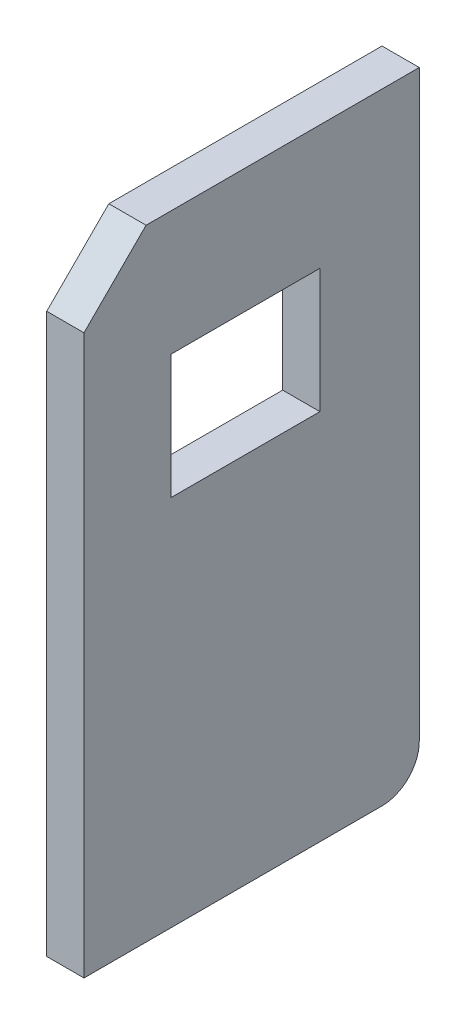
from build123d import *

# Parameters (mm, degrees)
EXTRUDE_1_DEPTH     = 3
FILLET_1_R          = 3
SKETCH_2_W          = 12
SKETCH_2_H          = 10
CUT_EXTRUDE_1_DEPTH = 57.903426962


with BuildPart() as part:
    # 草图1 → 凸台-拉伸1 (new body)
    with BuildSketch(Plane(origin=(0, 0, 0), x_dir=(0, 0, -1), z_dir=(1, 0, 0))):
        Polygon((-22, 50), (-27, 45), (-27, 0), (0, 0), (0, 50), align=None)
    extrude(amount=EXTRUDE_1_DEPTH)

    # 圆角1
    fillet_1_edges = [part.edges().sort_by_distance(p)[0] for p in [
        (1.5, 0, 0),
    ]]
    fillet(fillet_1_edges, radius=FILLET_1_R)

    # 草图2 → 切除-拉伸1 (cut, through all)
    with BuildSketch(Plane(origin=(3, 0, 0), x_dir=(0, 0, -1), z_dir=(1, 0, 0))):
        with Locations((-14, 35)):
            Rectangle(SKETCH_2_W, SKETCH_2_H)
    extrude(amount=-CUT_EXTRUDE_1_DEPTH, mode=Mode.SUBTRACT)


solid = part.part
